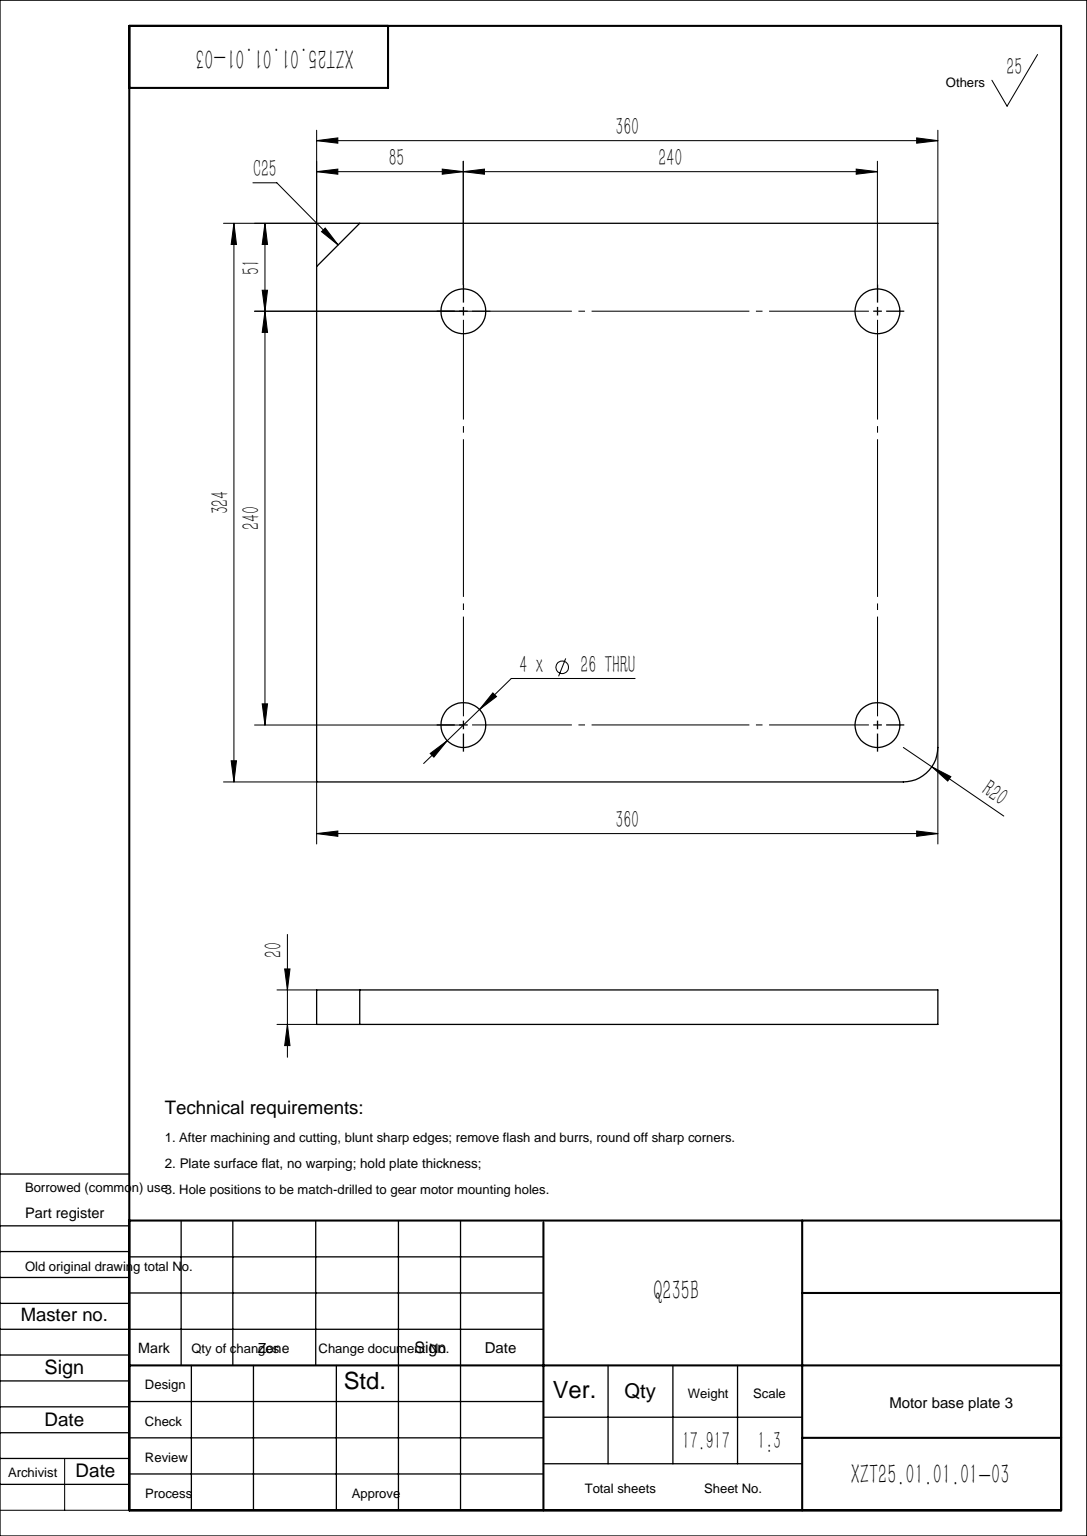
SolidWorks part; units mm, degrees
material "Q235B"
ref_plane "Front Plane" through (0, 0, 0) normal (0, 0, 1) x (1, 0, 0)
ref_plane "Top Plane" through (0, 0, 0) normal (0, 1, 0) x (1, 0, 0)
ref_plane "Right Plane" through (0, 0, 0) normal (1, 0, 0) x (0, 0, -1)
sketch "Sketch1" plane through (0, 0, 0) normal (0, 0, 1) x (1, 0, 0)
  line L1 (0, 0) -> (360, 0)
  line L2 (0, 0) -> (0, 324)
  line L3 (0, 324) -> (360, 324)
  line L4 (360, 0) -> (360, 324)
  dimension "D1" = 324
  dimension "D2" = 360
extrude "Boss-Extrude1" add sketch "Sketch1" along normal mid plane 20
chamfer "Chamfer1" distance 25 angle 45 1 edges at (0, 324, 0)
fillet "Fillet1" radius 20 1 edges at (360, 0, 0)
hole_wizard "Ø25.0 (25) Diameter Hole1" positions "Sketch2" profile "Sketch3" hole size "Ø25.0" standard "GB" end condition up to next
sketch "Sketch2" plane through (0, 0, 10) normal (0, 0, 1) x (1, 0, 0)
  line L0 (85, 33) -> (325, 33) construction
  line L1 (85, 33) -> (85, 273) construction
  line L2 (360, 324) -> (25, 324) construction
  line L3 (0, 299) -> (0, 0) construction
  point P0 (85, 33)
  point P7 (325, 33)
  point P8 (325, 273)
  point P9 (85, 273)
  dimension "D3" = 90
  dimension "D4" = 240
  dimension "D5" = 240
  dimension "D6" = 51
  dimension "D7" = 85
  dimension "D1" = 2
  dimension "D2" = 2
sketch "Sketch3" plane through (85, 33, 10) normal (1, 0, 0) x (0, -1, 0)
  line L0 (0, 0) -> (0, 20)
  line L1 (0, 20) -> (13, 20)
  line L2 (13, 20) -> (13, 0)
  line L5 (13, 0) -> (0, 0)
  line L11 (0, -6.35) -> (0, 107.95) construction
  dimension "通孔孔直径" = 26
  dimension "通孔孔深度" = 20
